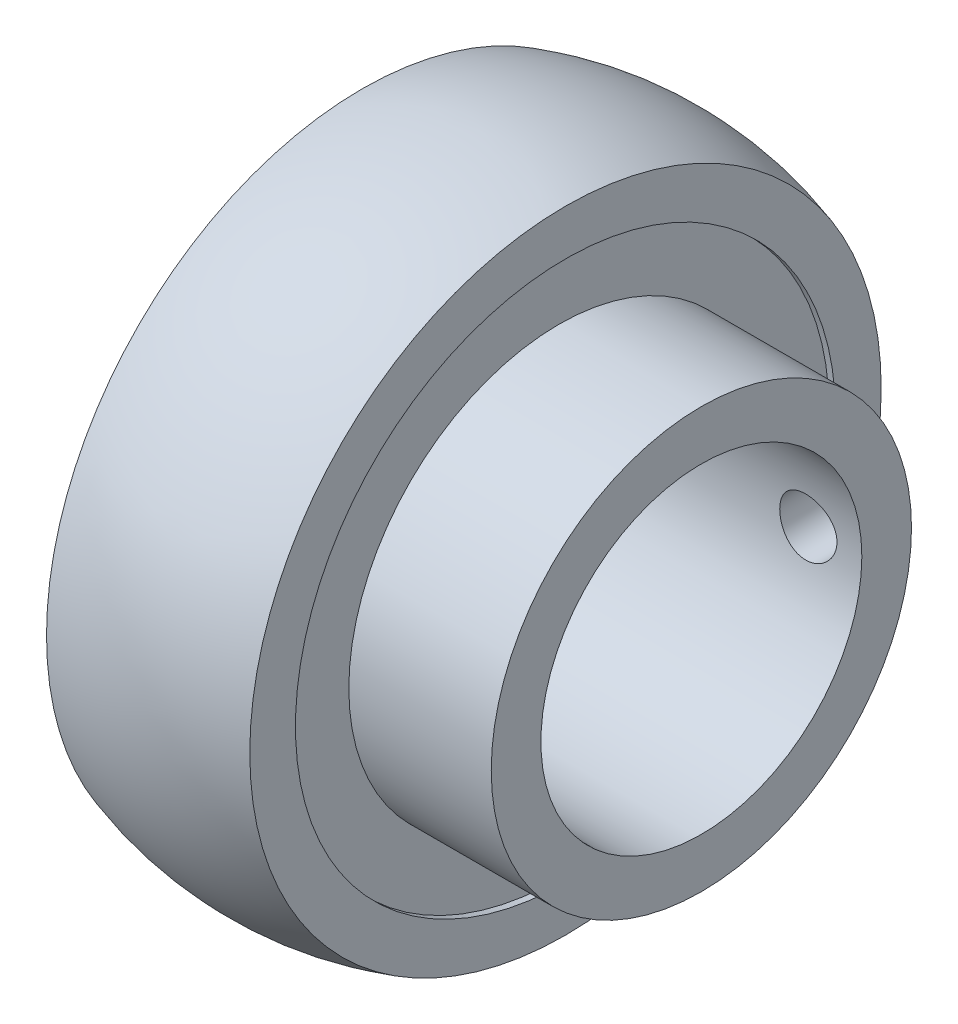
from build123d import *

# Parameters (mm, degrees)
SKETCH_2_W               = 38.1
SKETCH_2_H               = 4.64
PATTERN_CIRCULAR_1_COUNT = 4
SKETCH_5_W               = 0.2
SKETCH_5_H               = 6.09
SKETCH_4_W               = 2.67525
SKETCH_4_H               = 6.94
SKETCH_6_W               = 1.25
SKETCH_6_H               = 6.76


with BuildPart() as part:
    # 草图3 → Revolve 502 (revolve)
    with BuildSketch(Plane(origin=(0, 0, 0), x_dir=(0, 0, -1), z_dir=(1, 0, 0))):
        with BuildLine():
            Line((0, 18.44), (0, 27.56))
            ThreePointArc((0, 27.56), (4.56, 23), (0, 18.44))
        make_face()
    revolve_502 = revolve(axis=Axis((0, 0, 0), (0, 1, 0)))

    # 草图2 → 凸台-旋转3 (revolve)
    with BuildSketch(Plane.XY, mode=Mode.PRIVATE) as revolve_3_sk:
        with BuildLine():
            Line((-9.5, 25.24), (9.5, 25.24))
            Line((9.5, 25.24), (9.5, 29.508473359))
            ThreePointArc((9.5, 29.508473359), (0, 31), (-9.5, 29.508473359))
            Line((-9.5, 29.508473359), (-9.5, 25.24))
        make_face()
        with Locations((3.15, 17.32)):
            Rectangle(SKETCH_2_W, SKETCH_2_H)
    revolve(revolve_3_sk.sketch.rotate(Axis((0, 0, 0), (-1, 0, 0)), 90), axis=Axis((0, 0, 0), (-1, 0, 0)))

    # 阵列(圆周)1: Revolve 502 ×4 about axis
    pattern_circular_1_axis = Axis((0, 0, 0), (1, 0, 0))
    for i in range(1, PATTERN_CIRCULAR_1_COUNT):
        add(revolve_502.rotate(pattern_circular_1_axis, i * 360 / PATTERN_CIRCULAR_1_COUNT))

    # 草图5 → 凸台-旋转4 (revolve)
    with BuildSketch(Plane.XY, mode=Mode.PRIVATE) as revolve_4_sk:
        with Locations((-8.8, 22.695)):
            Rectangle(SKETCH_5_W, SKETCH_5_H)
        with Locations((8.8, 22.695)):
            Rectangle(SKETCH_5_W, SKETCH_5_H)
    revolve(revolve_4_sk.sketch.rotate(Axis((0, 0, 0), (-1, 0, 0)), 90), axis=Axis((0, 0, 0), (-1, 0, 0)))

    # 草图4 → 切除-旋转1 (revolve, cut)
    with BuildSketch(Plane(origin=(0, 0, 0), x_dir=(1, 0, 0), z_dir=(0, 1, 0)), mode=Mode.PRIVATE) as cut_revolve_1_sk:
        with Locations((18.537625, 16.47)):
            Rectangle(SKETCH_4_W, SKETCH_4_H)
    revolve(cut_revolve_1_sk.sketch.rotate(Axis((17.2, 0, -19.94), (0, 0, 1)), 180), axis=Axis((17.2, 0, -19.94), (0, 0, 1)), mode=Mode.SUBTRACT)

    # 草图6 → 切除-旋转2 (revolve, cut)
    with BuildSketch(Plane(origin=(0, 0, 0), x_dir=(1, 0, 0), z_dir=(0, 1, 0)), mode=Mode.PRIVATE) as cut_revolve_2_sk:
        with Locations((5.625, 28.12)):
            Rectangle(SKETCH_6_W, SKETCH_6_H)
    revolve(cut_revolve_2_sk.sketch.rotate(Axis((5, 0, -31.5), (0, 0, 1)), 180), axis=Axis((5, 0, -31.5), (0, 0, 1)), mode=Mode.SUBTRACT)


solid = part.part
